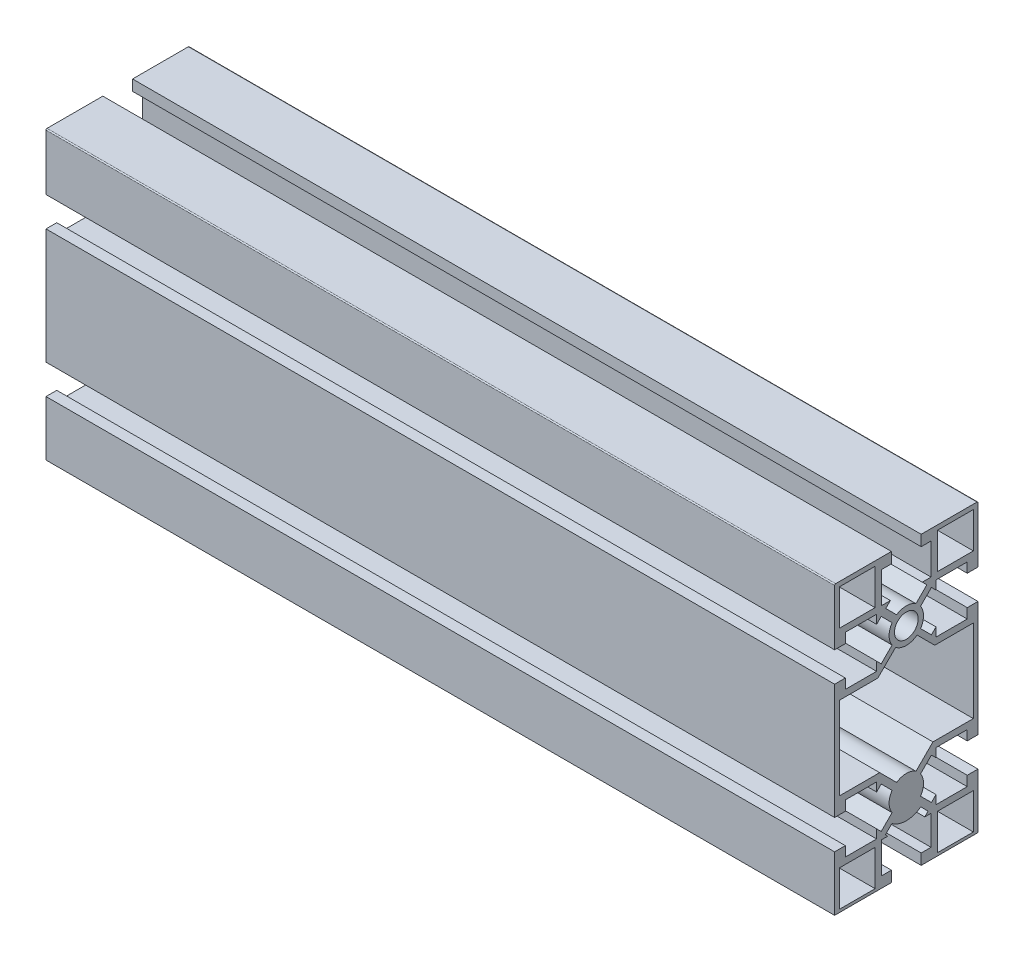
SolidWorks part; units mm, degrees
material "6063-T5"
ref_plane "Front Plane" through (0, 0, 0) normal (0, 0, 1) x (1, 0, 0)
ref_plane "Top Plane" through (0, 0, 0) normal (0, 1, 0) x (1, 0, 0)
ref_plane "Right Plane" through (0, 0, 0) normal (1, 0, 0) x (0, 0, -1)
sketch "Sketch2" plane through (0, 0, 0) normal (0, 1, 0) x (1, 0, 0)
  line L0 (-251.1276, -4.6291) -> (-31.1276, -4.6291)
  dimension "D1" = 220
other "Aluminum profile 40 X 80L X R0.3(1)"
ref_plane "Plane1" through (-251.1276, 0, 4.6291) normal (1, 0, 0) x (0, 0, -1)
sketch "Sketch13" plane through (-251.1276, 0, 4.6291) normal (1, 0, 0) x (0, 0, -1)
  line L0 (0, 0) -> (0, 16.3773) construction
  line L1 (0, 0) -> (-13.9576, 13.9576) construction
  line L2 (-19.7, 20) -> (-4.15, 20)
  line L3 (-20, 19.7) -> (-20, 4.15)
  line L4 (-18.7, -8.7) -> (-18.7, -31.8)
  line L5 (20, 19.7) -> (20, 4.15)
  line L6 (-8.2836, 6.9) -> (-8.2836, 4.4444)
  line L7 (-8.2836, 4.4444) -> (-7.0004, 5.7276)
  line L8 (-7.0004, 5.7276) -> (-3.9703, 2.6975)
  line L9 (0, 0) -> (20.7093, 0) construction
  line L10 (-4.4444, 8.2836) -> (-5.7276, 7.0004)
  line L11 (-6.9, 8.2836) -> (-4.4444, 8.2836)
  line L12 (-5.7276, 7.0004) -> (-2.6975, 3.9703)
  line L13 (8.2836, 6.9) -> (8.2836, 4.4444)
  line L14 (8.2836, 4.4444) -> (7.0004, 5.7276)
  line L15 (-4.15, 20) -> (-4.15, 17)
  line L16 (-18.7, 18.7) -> (-8.7, 18.7)
  line L17 (-18.7, 18.7) -> (-18.7, 8.7)
  line L18 (-18.7, 8.7) -> (-8.7, 8.7)
  line L19 (-8.7, 18.7) -> (-8.7, 8.7)
  line L20 (-6.9, 17) -> (-4.15, 17)
  line L21 (-6.9, 17) -> (-6.9, 8.2836)
  line L22 (7.0004, 5.7276) -> (3.9703, 2.6975)
  line L23 (6.9, 17) -> (6.9, 8.2836)
  line L24 (4.15, 20) -> (4.15, 17)
  line L25 (4.15, 20) -> (19.7, 20)
  line L26 (4.15, 17) -> (6.9, 17)
  line L27 (8.7, 18.7) -> (8.7, 8.7)
  line L28 (18.7, 8.7) -> (8.7, 8.7)
  line L29 (18.7, 18.7) -> (18.7, 8.7)
  line L30 (18.7, 18.7) -> (8.7, 18.7)
  line L31 (17, 6.9) -> (8.2836, 6.9)
  line L32 (17, 6.9) -> (17, 4.15)
  line L33 (20, 4.15) -> (17, 4.15)
  line L34 (18.7, -8.7) -> (18.7, -31.8)
  line L35 (17, -6.9) -> (8.2836, -6.9)
  line L36 (17, -4.15) -> (17, -6.9)
  line L37 (20, -4.15) -> (17, -4.15)
  line L38 (-2.1492, -20) -> (7.8508, -20) construction
  line L39 (-17, -44.65) -> (-20, -44.65)
  line L40 (-18.7, -49.2) -> (-18.7, -59.2)
  line L41 (-2.6975, -36.5297) -> (-7.4272, -31.8)
  line L42 (2.6975, -36.5297) -> (7.4272, -31.8)
  line L43 (-18.7, -31.8) -> (-7.4272, -31.8)
  line L44 (7.4272, -31.8) -> (18.7, -31.8)
  line L45 (-17, -6.9) -> (-8.2836, -6.9)
  line L46 (-17, -6.9) -> (-17, -4.15)
  line L47 (-20, -4.15) -> (-17, -4.15)
  line L48 (5.7276, 7.0004) -> (2.6975, 3.9703)
  line L49 (-17, 6.9) -> (-8.2836, 6.9)
  line L50 (-17, 4.15) -> (-17, 6.9)
  line L51 (-20, 4.15) -> (-17, 4.15)
  line L52 (-18.7, -8.7) -> (-7.9272, -8.7)
  line L53 (-20, -4.15) -> (-20, -36.35)
  line L54 (20, -4.15) -> (20, -36.35)
  line L55 (-7.9272, -8.7) -> (-2.9857, -3.7584)
  line L56 (18.7, -8.7) -> (7.9272, -8.7)
  line L57 (7.9272, -8.7) -> (2.9857, -3.7584)
  line L65 (4.4444, 8.2836) -> (5.7276, 7.0004)
  line L66 (6.9, 8.2836) -> (4.4444, 8.2836)
  line L70 (7.0004, -5.7276) -> (3.9703, -2.6975)
  line L71 (8.2836, -4.4444) -> (7.0004, -5.7276)
  line L72 (8.2836, -6.9) -> (8.2836, -4.4444)
  line L73 (-8.2836, -6.9) -> (-8.2836, -4.4444)
  line L74 (-8.2836, -4.4444) -> (-7.0004, -5.7276)
  line L75 (-7.0004, -5.7276) -> (-3.9703, -2.6975)
  line L85 (-17, -33.6) -> (-8.2836, -33.6)
  line L86 (-17, -36.35) -> (-17, -33.6)
  line L87 (-20, -36.35) -> (-17, -36.35)
  line L88 (-8.2836, -33.6) -> (-8.2836, -36.0556)
  line L89 (-8.2836, -36.0556) -> (-7.0004, -34.7724)
  line L90 (-7.0004, -34.7724) -> (-3.9703, -37.8025)
  line L103 (7.0004, -34.7724) -> (3.9703, -37.8025)
  line L104 (8.2836, -36.0556) -> (7.0004, -34.7724)
  line L105 (8.2836, -33.6) -> (8.2836, -36.0556)
  line L106 (17, -33.6) -> (8.2836, -33.6)
  line L108 (20, -36.35) -> (17, -36.35)
  line L114 (-17, -47.4) -> (-8.2836, -47.4)
  line L115 (-17, -47.4) -> (-17, -44.65)
  line L116 (-7.0004, -46.2276) -> (-3.9703, -43.1975)
  line L117 (-8.2836, -44.9444) -> (-7.0004, -46.2276)
  line L118 (-8.2836, -47.4) -> (-8.2836, -44.9444)
  line L119 (-5.1515, -48.2836) -> (-5.8311, -47.6039)
  line L120 (-6.9, -48.2836) -> (-5.1515, -48.2836)
  line L121 (-5.8311, -47.6039) -> (-4.0226, -45.7954)
  line L122 (-6.9, -57) -> (-6.9, -48.2836)
  line L123 (-8.7, -59.2) -> (-8.7, -49.2)
  line L124 (-18.7, -49.2) -> (-8.7, -49.2)
  line L125 (-20, -44.65) -> (-20, -60)
  line L126 (-18.7, -59.2) -> (-8.7, -59.2)
  line L127 (-20, -60) -> (-4.15, -60)
  line L128 (-4.15, -60) -> (-4.15, -57)
  line L129 (-4.15, -57) -> (-6.9, -57)
  line L130 (4.15, -60) -> (4.15, -57)
  line L131 (6.9, -57) -> (4.15, -57)
  line L132 (6.9, -57) -> (6.9, -48.7836)
  line L133 (6.9, -48.7836) -> (5.1515, -48.7836)
  line L134 (5.1515, -48.7836) -> (6.0811, -47.8539)
  line L135 (6.0811, -47.8539) -> (4.0226, -45.7954)
  line L136 (7.0004, -46.2276) -> (3.9703, -43.1975)
  line L137 (8.2836, -44.9444) -> (7.0004, -46.2276)
  line L138 (8.2836, -47.4) -> (8.2836, -44.9444)
  line L139 (17, -47.4) -> (8.2836, -47.4)
  line L140 (17, -44.65) -> (17, -47.4)
  line L141 (20, -44.65) -> (17, -44.65)
  line L142 (20, -44.65) -> (20, -60)
  line L143 (18.7, -59.2) -> (18.7, -49.2)
  line L144 (18.7, -49.2) -> (8.7, -49.2)
  line L145 (8.7, -59.2) -> (8.7, -49.2)
  line L146 (18.7, -59.2) -> (8.7, -59.2)
  line L147 (17, -33.6) -> (17, -36.35)
  line L148 (4.15, -60) -> (20, -60)
  line L149 (-20, -20.8) -> (-20, -36.35) [skipped]
  line L150 (-19.7, -20.5) -> (-4.15, -20.5) [skipped]
  line L152 (6.9, -17) -> (4.15, -17) [skipped]
  line L154 (4.15, -20) -> (4.15, -17) [skipped]
  line L156 (-4.15, -17) -> (-6.9, -17) [skipped]
  line L158 (-4.15, -20) -> (-4.15, -17) [skipped]
  line L162 (-18.7, -21.8) -> (-8.7, -21.8) [skipped]
  line L163 (-6.9, -23.5) -> (-4.15, -23.5) [skipped]
  line L164 (-4.15, -20.5) -> (-4.15, -23.5) [skipped]
  line L165 (4.15, -20.5) -> (4.15, -23.5) [skipped]
  line L166 (4.15, -23.5) -> (6.9, -23.5) [skipped]
  line L167 (18.7, -21.8) -> (8.7, -21.8) [skipped]
  line L168 (4.15, -20.5) -> (19.7, -20.5) [skipped]
  line L170 (20, -20.8) -> (20, -36.35) [skipped]
  line L171 (-18.7, -21.8) -> (-18.7, -31.8) [skipped]
  line L172 (-8.7, -21.8) -> (-8.7, -31.8) [skipped]
  line L173 (-6.9, -23.5) -> (-6.9, -32.2164) [skipped]
  line L176 (-6.9, -17) -> (-6.9, -8.2836) [skipped]
  line L178 (6.9, -17) -> (6.9, -8.2836) [skipped]
  line L180 (8.7, -21.8) -> (8.7, -31.8) [skipped]
  line L181 (6.9, -23.5) -> (6.9, -32.2164) [skipped]
  line L183 (18.7, -21.8) -> (18.7, -31.8) [skipped]
  line L184 (-4.4444, -32.2164) -> (-5.7276, -33.4996) [skipped]
  line L185 (-6.9, -32.2164) -> (-4.4444, -32.2164) [skipped]
  line L186 (6.9, -32.2164) -> (4.4444, -32.2164) [skipped]
  line L187 (4.4444, -32.2164) -> (5.7276, -33.4996) [skipped]
  line L188 (5.7276, -33.4996) -> (2.6975, -36.5297) [skipped]
  line L189 (-5.7276, -33.4996) -> (-2.6975, -36.5297) [skipped]
  line L190 (-18.7, -31.8) -> (-8.7, -31.8) [skipped]
  line L191 (18.7, -31.8) -> (8.7, -31.8) [skipped]
  line L193 (-4.4444, -8.2836) -> (-5.7276, -7.0004) [skipped]
  line L195 (-6.9, -8.2836) -> (-4.4444, -8.2836) [skipped]
  line L197 (6.9, -8.2836) -> (4.4444, -8.2836) [skipped]
  line L199 (4.4444, -8.2836) -> (5.7276, -7.0004) [skipped]
  line L201 (5.7276, -7.0004) -> (2.6975, -3.9703) [skipped]
  line L204 (-5.7276, -7.0004) -> (-2.6975, -3.9703) [skipped]
  circle A0 centre (0, 0) radius 3.3
  arc A1 (-3.9703, 2.6975) -> (-3.9703, -2.6975) centre (0, 0) ccw
  arc A2 (-2.9857, -3.7584) -> (2.9857, -3.7584) centre (0, 0) ccw
  arc A3 (3.9703, -2.6975) -> (3.9703, 2.6975) centre (0, 0) ccw
  arc A4 (2.6975, 3.9703) -> (-2.6975, 3.9703) centre (0, 0) ccw
  arc A6 (2.6975, -36.5297) -> (-2.6975, -36.5297) centre (0, -40.5) ccw
  arc A7 (-3.9703, -37.8025) -> (-3.9703, -43.1975) centre (0, -40.5) ccw
  arc A8 (-19.7, 20) -> (-20, 19.7) centre (-19.7, 19.7) ccw
  arc A9 (19.7, 20) -> (20, 19.7) centre (19.7, 19.7) cw
  arc A12 (-4.0226, -45.7954) -> (4.0226, -45.7954) centre (0, -40.5) ccw
  arc A13 (3.9703, -43.1975) -> (3.9703, -37.8025) centre (0, -40.5) ccw
  arc A14 (-19.7, -20.5) -> (-20, -20.8) centre (-19.7, -20.8) ccw [skipped]
  point P65 (0, 0)
  dimension "D2" = 4.8
  dimension "D3" = 6.6
  dimension "D4" = 40
  dimension "D5" = 3
  dimension "D6" = 1.8
  dimension "D7" = 1.3
  dimension "D8" = 13.8
  dimension "D10" = 9
  dimension "D11" = 10
  dimension "D12" = 80
  dimension "D13" = 8.3
  dimension "D14" = 0.3
  dimension "D15" = 40.5
  dimension "D9" = 1.3
  dimension "D16" = 1.8
